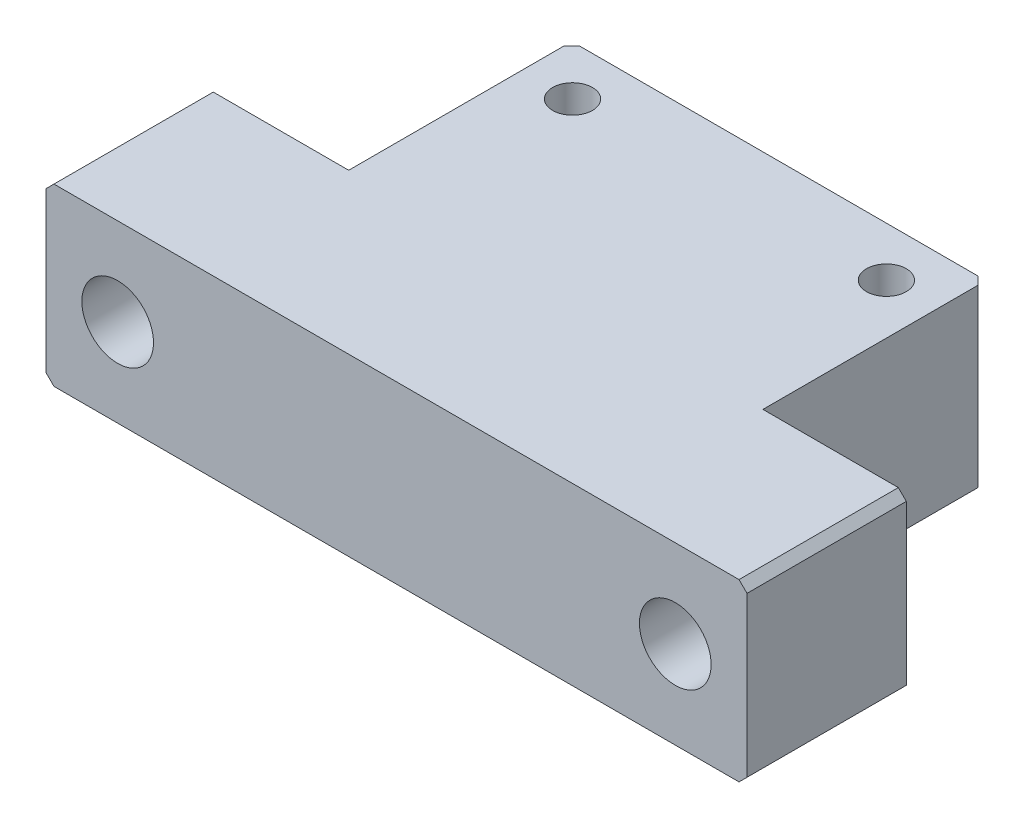
from build123d import *

# Parameters (mm, degrees)
SKETCH1_W                                            = 44
SKETCH1_H                                            = 11
BOSS_EXTRUDE1_DEPTH                                  = 24
SKETCH2_W                                            = 9
SKETCH2_H                                            = 14
CUT_EXTRUDE1_DEPTH                                   = 35.365680555
CBORE_FOR_M4_HEXAGON_SOCKET_HEAD_CAP_SCR_D           = 4.5
CBORE_FOR_M4_HEXAGON_SOCKET_HEAD_CAP_SCR_CBORE_D     = 8
CBORE_FOR_M4_HEXAGON_SOCKET_HEAD_CAP_SCR_CBORE_DEPTH = 4.6
M3_TAPPED_HOLE1_D                                    = 2.5
CHAMFER1_SIZE                                        = 0.5
CHAMFER2_SIZE                                        = 0.5


with BuildPart() as part:
    # Sketch1 → Boss-Extrude1 (new body)
    with BuildSketch(Plane.XY):
        Rectangle(SKETCH1_W, SKETCH1_H)
    extrude(amount=BOSS_EXTRUDE1_DEPTH)

    # Sketch2 → Cut-Extrude1 (cut, through all)
    with BuildSketch(Plane(origin=(0, 5.5, 0), x_dir=(1, 0, 0), z_dir=(0, 1, 0))):
        with Locations((-17.5, -7)):
            Rectangle(SKETCH2_W, SKETCH2_H)
        with Locations((17.5, -7)):
            Rectangle(SKETCH2_W, SKETCH2_H)
    extrude(amount=-CUT_EXTRUDE1_DEPTH, mode=Mode.SUBTRACT)

    # CBORE for M4 Hexagon socket head cap screws1 (through all)
    with Locations(Plane(origin=(0, 0, 14), x_dir=(-1, 0, 0), z_dir=(0, 0, -1))):
        with Locations((-17.5, 0), (17.5, 0)):
            CounterBoreHole(CBORE_FOR_M4_HEXAGON_SOCKET_HEAD_CAP_SCR_D / 2, CBORE_FOR_M4_HEXAGON_SOCKET_HEAD_CAP_SCR_CBORE_D / 2, CBORE_FOR_M4_HEXAGON_SOCKET_HEAD_CAP_SCR_CBORE_DEPTH)

    # M3 Tapped Hole1 (through all)
    with Locations(Plane(origin=(0, 5.5, 0), x_dir=(1, 0, 0), z_dir=(0, 1, 0))):
        with Locations((9.85, -3.1), (-9.85, -3.1)):
            Hole(M3_TAPPED_HOLE1_D / 2)

    # Chamfer1
    chamfer1_edges = [part.edges().sort_by_distance(p)[0] for p in [
        (22, -5.5, 19),
        (-22, -5.5, 19),
        (-22, 5.5, 19),
        (22, 5.5, 19),
    ]]
    chamfer(chamfer1_edges, length=CHAMFER1_SIZE)

    # Chamfer2
    chamfer2_edges = [part.edges().sort_by_distance(p)[0] for p in [
        (-13, 0, 0),
        (13, 0, 0),
    ]]
    chamfer(chamfer2_edges, length=CHAMFER2_SIZE)


solid = part.part
